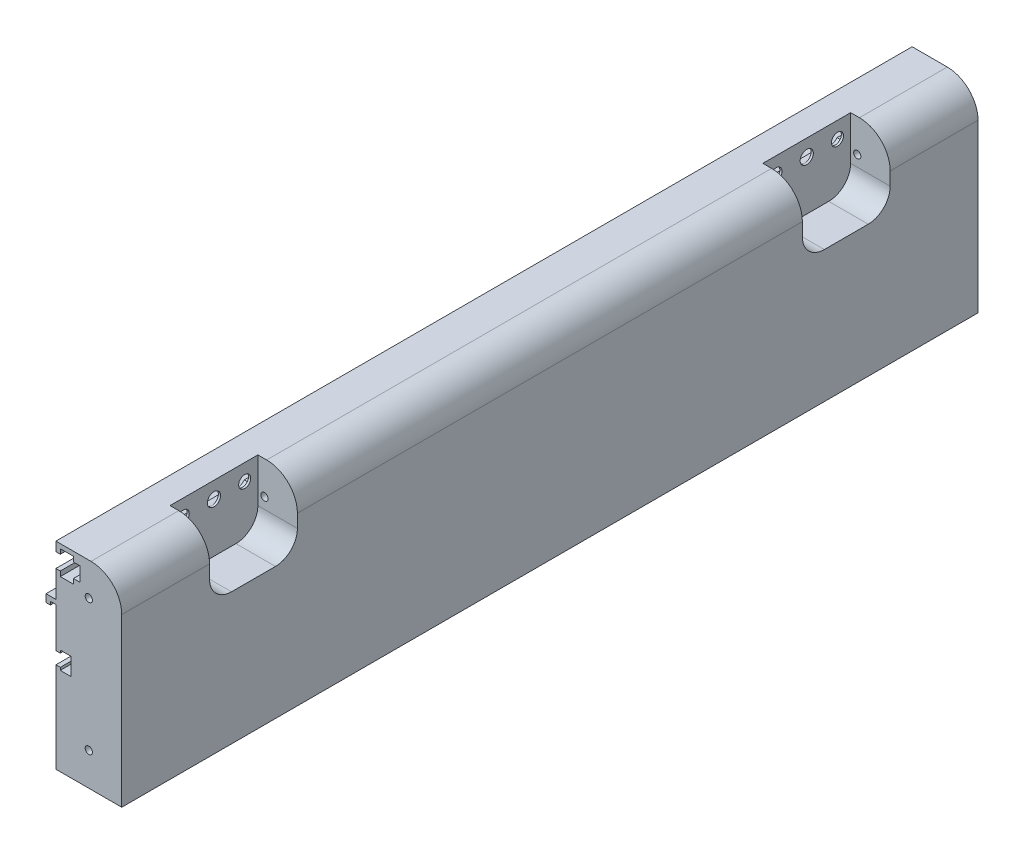
SolidWorks part; units mm, degrees
ref_plane "Front Plane" through (0, 0, 0) normal (0, 0, 1) x (1, 0, 0)
ref_plane "Top Plane" through (0, 0, 0) normal (0, 1, 0) x (1, 0, 0)
ref_plane "Right Plane" through (0, 0, 0) normal (1, 0, 0) x (0, 0, -1)
sketch "Sketch1" plane through (0, 0, 0) normal (0, 0, 1) x (1, 0, 0)
  line L0 (0, 0) -> (0, 41.2)
  line L1 (0, 90) -> (16, 90)
  line L4 (0, 67) -> (-4.5, 67)
  line L5 (-4.5, 67) -> (-4.5, 63.5)
  line L6 (-4.5, 63.5) -> (-2.5, 63.5)
  line L7 (-2.5, 63.5) -> (-2.5, 65)
  line L8 (-2.5, 65) -> (0, 65)
  line L9 (0, 46.8) -> (2, 46.8)
  line L10 (2, 46.8) -> (2, 48)
  line L11 (2, 48) -> (7, 48)
  line L12 (7, 48) -> (7, 40)
  line L13 (7, 40) -> (2, 40)
  line L14 (2, 40) -> (2, 41.2)
  line L15 (2, 41.2) -> (0, 41.2)
  line L16 (7, 44) -> (0, 44) construction
  line L17 (0, 46.8) -> (0, 65)
  line L27 (0, 85.8) -> (2, 85.8)
  line L28 (2, 85.8) -> (2, 88)
  line L29 (2, 88) -> (8, 88)
  line L30 (8, 88) -> (8, 85.75)
  line L31 (8, 77) -> (2, 77)
  line L32 (2, 77) -> (2, 79.2)
  line L33 (2, 79.2) -> (0, 79.2)
  line L34 (0, 85.8) -> (0, 90)
  line L42 (30, 76) -> (30, 0)
  line L50 (30, 0) -> (0, 0)
  line L51 (0, 67) -> (0, 79.2)
  line L52 (11, 82.5) -> (0, 82.5) construction
  line L53 (0, 82.5) -> (0, 85.8) construction
  line L54 (8, 85.75) -> (11, 85.75)
  line L55 (11, 85.75) -> (11, 79.25)
  line L56 (8, 79.25) -> (11, 79.25)
  line L57 (8, 79.25) -> (8, 77)
  line L58 (15, 75) -> (15, 15) construction
  arc A0 (16, 90) -> (30, 76) centre (16, 76) cw
  circle A1 centre (15, 75) radius 1.65
  circle A2 centre (15, 15) radius 1.65
  point P68 (11, 82.5)
  point P69 (1, 41.2)
  dimension "D3" = 14
  dimension "D30" = 3.3
  dimension "D31" = 60
  dimension "D34" = 3.3
  dimension "D1" = 90
  dimension "D2" = 30
  dimension "D4" = 23
  dimension "D5" = 4.5
  dimension "D6" = 3.5
  dimension "D7" = 2
  dimension "D8" = 2
  dimension "D9" = 46
  dimension "D10" = 5.6
  dimension "D11" = 2
  dimension "D12" = 5
  dimension "D13" = 8
  dimension "D14" = 7
  dimension "D15" = 6.6
  dimension "D16" = 6
  dimension "D17" = 2
  dimension "D18" = 2
  dimension "D19" = 11
  dimension "D32" = 3
  dimension "D33" = 6.5
  dimension "D35" = 15
  dimension "D36" = 15
extrude "Boss-Extrude1" add sketch "Sketch1" along normal mid plane 390
sketch "Sketch2" plane through (0, 0, 0) normal (-1, 0, 0) x (0, 0, 1)
  line L0 (0, 0) -> (0, 90) construction
  line L1 (195, 0) -> (-195, 0) construction
  line L2 (195, 90) -> (-195, 90) construction
  line L3 (-155, 46.8) -> (-155, 41.2) construction
  line L4 (195, 46.8) -> (-195, 46.8) construction
  line L5 (195, 41.2) -> (-195, 41.2) construction
  line L6 (-195, 65) -> (-195, 46.8) construction
  circle A0 centre (-155, 44) radius 11
  circle A1 centre (155, 44) radius 11
  dimension "D1" = 22
  dimension "D2" = 40
extrude "Cut-Extrude1" cut sketch "Sketch2" against normal blind 7
sketch "Sketch3" plane through (0, 0, 0) normal (-1, 0, 0) x (0, 0, 1)
  line L0 (-135, 85.8) -> (-135, 79.2) construction
  line L1 (195, 79.2) -> (-195, 79.2) construction
  line L2 (-195, 88) -> (-195, 85.75) construction
  line L3 (195, 85.8) -> (-195, 85.8) construction
  line L4 (0, 0) -> (0, 41.2) construction
  line L5 (195, 0) -> (-195, 0) construction
  line L6 (144.3623, 41.2) -> (-144.3623, 41.2) construction
  line L7 (135, 85.8) -> (135, 79.2) construction
  circle A0 centre (-135, 82.5) radius 3
  circle A1 centre (135, 82.5) radius 3
  dimension "D1" = 6
  dimension "D2" = 60
extrude "Cut-Extrude2" cut sketch "Sketch3" against normal through all
hole_wizard "M4 Tapped Hole2" positions "Sketch6" profile "Sketch5" tap size "M4" standard "GB"
sketch "Sketch6" plane through (0, 90, 0) normal (0, 1, 0) x (1, 0, 0)
  line L0 (0, -235) -> (0, 235) construction
  line L1 (16, -235) -> (0, -235) construction
  point P0 (5, -200)
  point P3 (5, -210)
  point P11 (5, -220)
  point P13 (5, -230)
  dimension "D1" = 5
  dimension "D2" = 10
  dimension "D3" = 25
  dimension "D4" = 10
  dimension "D5" = 5
sketch "Sketch5" plane through (5, 90, 200) normal (1, 0, 0) x (0, 0, 1)
  line L0 (0, 0) -> (0, 36.202)
  line L1 (0, 36.202) -> (1.65, 36.202)
  line L2 (1.65, 36.202) -> (1.65, 0)
  line L5 (1.65, 0) -> (0, 0)
  line L11 (0, -6.35) -> (0, 107.95) construction
  dimension "通孔螺纹孔钻头直径" = 3.3
  dimension "通孔螺纹孔钻头深度" = 36.202
cosmetic thread "Hole thread line10" [suppressed] parameters "D2"=4
cosmetic thread "Hole thread line8" [suppressed] parameters "D2"=4
cosmetic thread "Hole thread line7" [suppressed] parameters "D2"=4
cosmetic thread "Hole thread line9" [suppressed] parameters "D2"=4
mirror "Mirror1" [suppressed] about plane through (0, 0, 0) normal (0, 0, 1)
sketch "Sketch9" plane through (30, 0, 0) normal (1, 0, 0) x (0, 0, -1)
  line L0 (-195, 90) -> (195, 90) construction
  line L1 (-155, 90) -> (-115, 90)
  line L2 (-155, 90) -> (-155, 70)
  line L3 (-145, 60) -> (-125, 60)
  line L4 (-115, 90) -> (-115, 70)
  line L5 (-135, 90) -> (-135, 60) construction
  line L6 (-195, 0) -> (-195, 76) construction
  arc A0 (-125, 60) -> (-115, 70) centre (-125, 70) ccw
  arc A1 (-155, 70) -> (-145, 60) centre (-145, 70) ccw
  point P12 (-115, 60)
  point P15 (-155, 60)
  dimension "D4" = 10
  dimension "D1" = 40
  dimension "D2" = 60
  dimension "D3" = 30
extrude "Cut-Extrude4" cut sketch "Sketch9" against normal offset from surface (18 mm away) 12 up to face at (0, 73.1, 0)
hole_wizard "M5 socket head cap screw type1" positions "Sketch10" profile "Sketch11" counterbore size "M5" standard "GB" end condition up to next
sketch "Sketch10" plane through (0, 0, 0) normal (-1, 0, 0) x (0, 0, 1)
  line L0 (135, 82.5) -> (121, 82.5) construction
  line L3 (135, 82.5) -> (149, 82.5) construction
  circle A0 centre (135, 82.5) radius 3 construction
  point P0 (149, 82.5)
  point P3 (121, 82.5)
  dimension "D2" = 14
  dimension "D1" = 14
sketch "Sketch11" plane through (0, 82.5, 149) normal (0, 1, 0) x (0, 0, 1)
  line L0 (0, 0) -> (0, 12.001)
  line L1 (0, 12.001) -> (2.75, 12.001)
  line L3 (2.75, 12.001) -> (2.75, 11)
  line L4 (2.75, 11) -> (5, 11)
  line L5 (5, 11) -> (5, 0)
  line L7 (5, 0) -> (0, 0)
  line L11 (0, -6.35) -> (0, 107.95) construction
  dimension "通孔孔直径" = 5.5
  dimension "通孔孔深度" = 12.001
  dimension "柱形沉头孔直径" = 10
  dimension "柱形沉头孔深度" = 11
mirror "Mirror2" about plane through (0, 0, 0) normal (0, 0, 1) of "M5 socket head cap screw type1", "Cut-Extrude2", "Cut-Extrude4"
